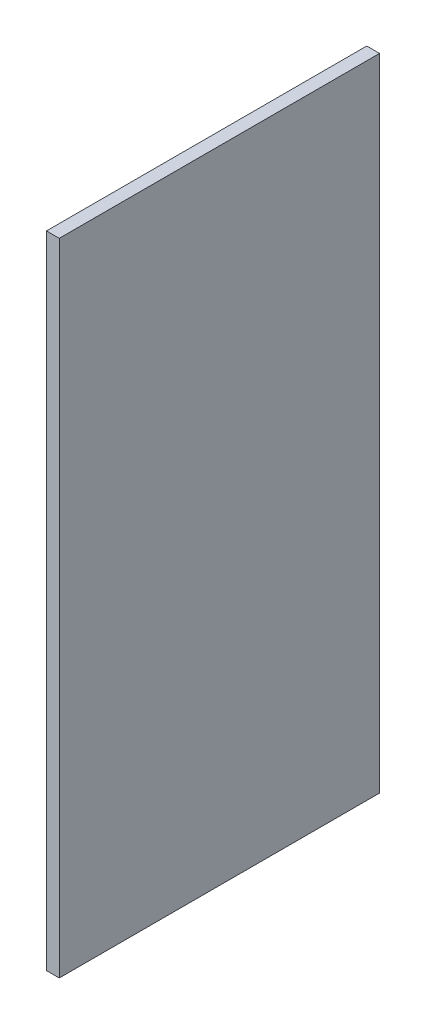
SolidWorks part; units mm, degrees
material "Q235"
ref_plane "前视基准面" through (0, 0, 0) normal (0, 0, 1) x (1, 0, 0)
ref_plane "上视基准面" through (0, 0, 0) normal (0, 1, 0) x (1, 0, 0)
ref_plane "右视基准面" through (0, 0, 0) normal (1, 0, 0) x (0, 0, -1)
sketch "草图1" plane through (0, 0, 0) normal (1, 0, 0) x (0, 0, -1)
  line L1 (0, 0) -> (100, 0)
  line L2 (0, 0) -> (0, 200)
  line L3 (0, 200) -> (100, 200)
  line L4 (100, 0) -> (100, 200)
  dimension "D1" = 200
  dimension "D2" = 100
extrude "凸台-拉伸1" add sketch "草图1" along normal blind 4
